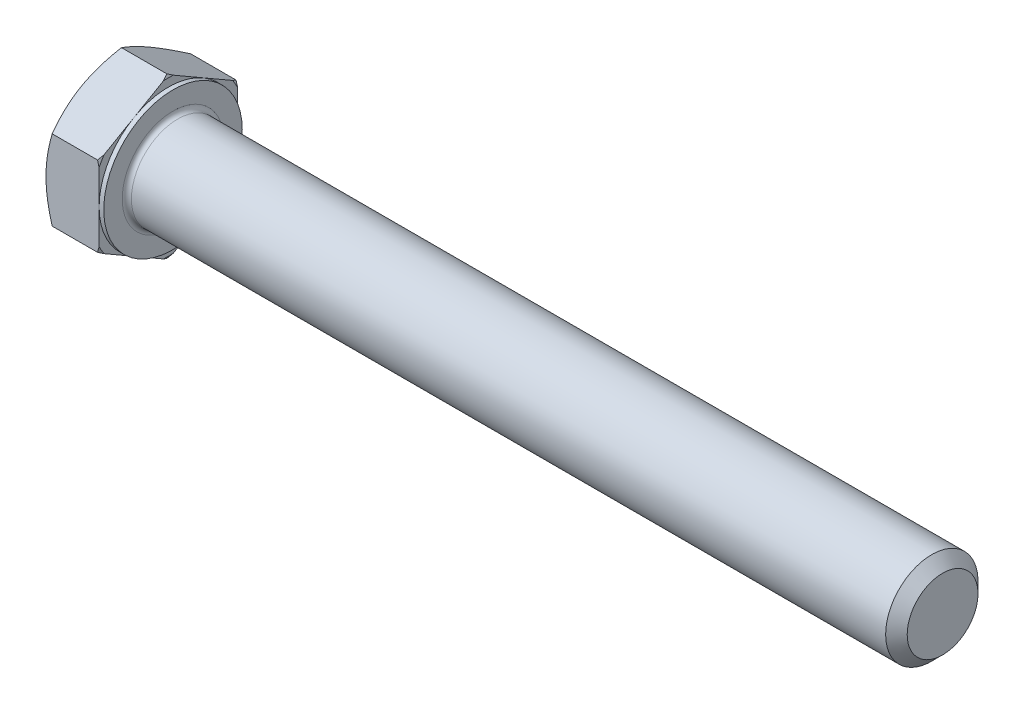
SolidWorks part; units mm, degrees
extrude "Base-extrude" add sketch "Sketch1" along normal blind 7.5
sketch "Sketch1" plane through (0, 0, 0) normal (1, 0, 0) x (0, 0, -1)
  line L0 (9, 5.1962) -> (9, -5.1962)
  line L1 (-9, 5.1962) -> (-9, -5.1962)
  line L2 (9, -5.1962) -> (0, -10.3923)
  line L3 (0, -10.3923) -> (-9, -5.1962)
  line L4 (9, 5.1962) -> (0, 10.3923)
  line L5 (0, 10.3923) -> (-9, 5.1962)
revolve "Cut-Revolve1" cut sketch "Sketch3" angle 360 about L6
sketch "Sketch3" plane through (0, 0, 0) normal (0, 0, 1) x (1, 0, 0)
  line L0 (0, 9) -> (3.6906, 15.3923)
  line L1 (0, 10.3923) -> (0, 5.1962) construction
  line L2 (3.6906, 15.3923) -> (3.6906, 20.3923)
  line L3 (3.6906, 20.3923) -> (-10, 20.3923)
  line L4 (-10, 20.3923) -> (-10, 9)
  line L5 (-10, 9) -> (0, 9)
  line L6 (0, 0) -> (99.06, 0) construction
  line L7 (7.5, 10.3923) -> (0, 10.3923) construction
ref_plane "Front" through (0, 0, 0) normal (0, 0, 1) x (1, 0, 0)
ref_plane "Top" through (0, 0, 0) normal (0, 1, 0) x (1, 0, 0)
ref_plane "Right" through (0, 0, 0) normal (1, 0, 0) x (0, 0, -1)
sketch "Sketch2" plane through (0, 0, 0) normal (0, 0, 1) x (1, 0, 0)
  line L0 (0, 5.1962) -> (0, -5.1962) construction
  line L1 (0, 0) -> (107.5, 0)
  line L2 (0, 0) -> (0, 6)
  line L3 (0, 6) -> (7.7917, 6)
  line L4 (107.5, 0) -> (107.5, 4.4845)
  line L5 (7.5, 10.3923) -> (7.5, 5.1962) construction
  line L7 (0, 0) -> (96.52, 0) construction
  line L8 (107.5, -4.4845) -> (7.7917, -6) construction
  line L9 (0, -6) -> (7.7917, -6) construction
  line L10 (9.25, 15.24) -> (9.25, -1.27) construction
  line L11 (77.5, 15.24) -> (77.5, -1.27) construction
  line L12 (7.5, 5.1962) -> (7.5, -5.1962) construction
  line L13 (7.7917, 6) -> (107.5, 6)
  line L14 (107.5, 6) -> (107.5, 4.4845)
revolve "Boss-Revolve1" add sketch "Sketch2" angle 360 about L7
cosmetic thread "Helix 1" parameters "Thread_length"=30, "Thread_minor"=8.969
sketch "Sketch5" plane through (0, 0, 0) normal (0, 0, 1) x (1, 0, 0)
  line L0 (7.5, 9) -> (3.8094, 15.3923)
  line L1 (7.5, 10.3923) -> (7.5, 5.1962) construction
  line L2 (3.8094, 15.3923) -> (3.8094, 20.3923)
  line L3 (3.8094, 20.3923) -> (13.8094, 20.3923)
  line L4 (13.8094, 20.3923) -> (13.8094, 9)
  line L5 (13.8094, 9) -> (7.5, 9)
  line L7 (7.5, 10.3923) -> (0.8038, 10.3923) construction
  line L8 (0, 0) -> (99.06, 0) construction
  line L9 (0, 0) -> (99.06, 0) construction
revolve "Cut-Revolve2" cut sketch "Sketch5" angle 360 about L8
sketch "Sketch4" plane through (0, 0, 0) normal (0, 0, 1) x (1, 0, 0)
  line L1 (7.5, 10.3923) -> (7.5, 5.1962) construction
  line L2 (7.5, 9) -> (6.9, 9)
  line L3 (7.5, 9) -> (7.5, 20.3923)
  line L4 (7.5, 20.3923) -> (6.9, 20.3923)
  line L5 (0, 0) -> (95.25, 0) construction
  line L6 (0, 0) -> (96.52, 0) construction
  line L7 (6.9, 9) -> (6.9, 20.3923)
  line L8 (6.6962, 10.3923) -> (0.8038, 10.3923) construction
revolve "Cut-Revolve3" cut sketch "Sketch4" angle 360 about L5
chamfer "Chamfer" distance 1.4 angle 45 1 edges at (107.5, 0, 6)
fillet "Fillet" radius 0.6 1 edges at (7.5, 0, -6)
sketch "Sketch6" plane through (0, 0, 0) normal (0, 0, 1) x (1, 0, 0)
  line L0 (77.5, -4.4845) -> (76.625, -6)
  line L1 (77.5, -4.4845) -> (78.375, -6)
  line L2 (78.375, -6) -> (78.375, -7.5)
  line L3 (-3.175, 0) -> (5.1513, 0) construction
  line L5 (78.375, -7.5) -> (76.625, -7.5)
  line L6 (76.625, -7.5) -> (76.625, -6)
revolve "Cut-Revolve4" [suppressed] cut sketch "Sketch6" angle 360 about L3
pattern_linear "LPattern1" [suppressed]
equation "\"D3@Sketch1\" = \"s@Sketch1\" / 2"
equation "\"D4@Sketch1\" = \"D3@Sketch1\""
equation "\"D5@Sketch1\" = \"D4@Sketch1\""
equation "\"Thread_minor@Helix 1\" = \"Minor_dia@Sketch2\""
equation "\"D1@Sketch3\" = \"s@Sketch1\" / 2"
equation "\"D1@Sketch5\" = \"s@Sketch1\" / 2"
equation "\"Head_ch_ang@Sketch5\" = \"Head_ch_ang@Sketch3\""
equation "\"D1@Sketch4\" = \"s@Sketch1\""
equation "\"Thread_length@Helix 1\" = ((sgn( (\"l@Sketch2\" - \"p@Sketch2\" ) - \"h@Sketch2\" )-1)*( (\"l@Sketch2\" - \"p@Sketch2\" ) - \"h@Sketch2\" ))/-2+ \"h@Sketch2\""
equation "\"Thread_minor@Sketch6\" = \"Minor_dia@Sketch2\""
equation "\"Diameter@Sketch6\" = \"m@Sketch2\""
equation "\"Overcut@Sketch6\" = \"m@Sketch2\" * 1.25"
equation "\"Start@Sketch6\" = \"k@Base-extrude\" + \"l@Sketch2\" - \"Thread_length@Helix 1\"  '---Non-countersunk---"
equation "\"Num_threads@LPattern1\" = int( \"Thread_length@Helix 1\" / \"p@Sketch2\" + 0.999 )  + 1"
equation "\"Advance@LPattern1\" = \"Thread_length@Helix 1\" /  (\"Num_threads@LPattern1\" - 1) 'relax it"
equation "\"Num_threads@LPattern1\" = \"Num_threads@LPattern1\" - sgn( \"Num_threads@LPattern1\" - 1) '---chamfered tips only---"
equation "\"Minor_dia@Sketch2\" = \"m@Sketch2\"-\"p@Sketch2\" * 1.732"
equation "\"D1@Chamfer\" = \"p@Sketch2\"*0.8"
